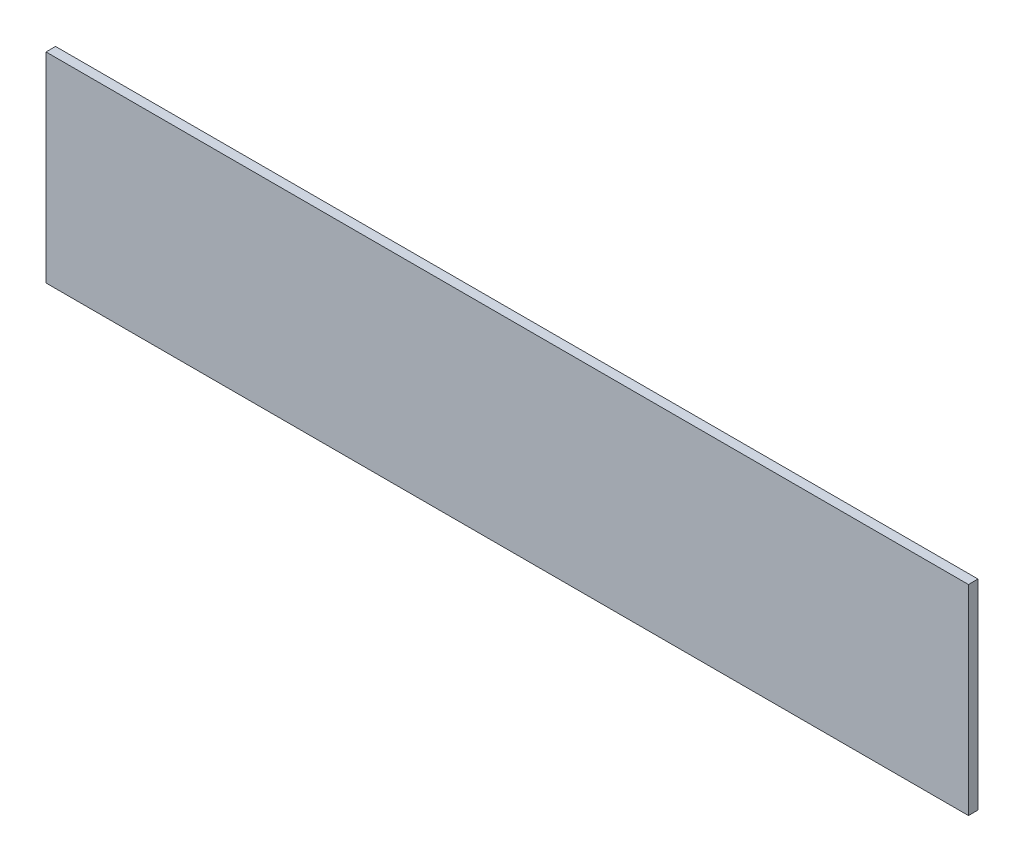
from build123d import *

# Parameters (mm, degrees)
SKETCH_1_W      = 484
SKETCH_1_H      = 105
EXTRUDE_1_DEPTH = 5


with BuildPart() as part:
    # 草图1 → 凸台-拉伸1 (new body)
    with BuildSketch(Plane.XY):
        Rectangle(SKETCH_1_W, SKETCH_1_H)
    extrude(amount=EXTRUDE_1_DEPTH)


solid = part.part
